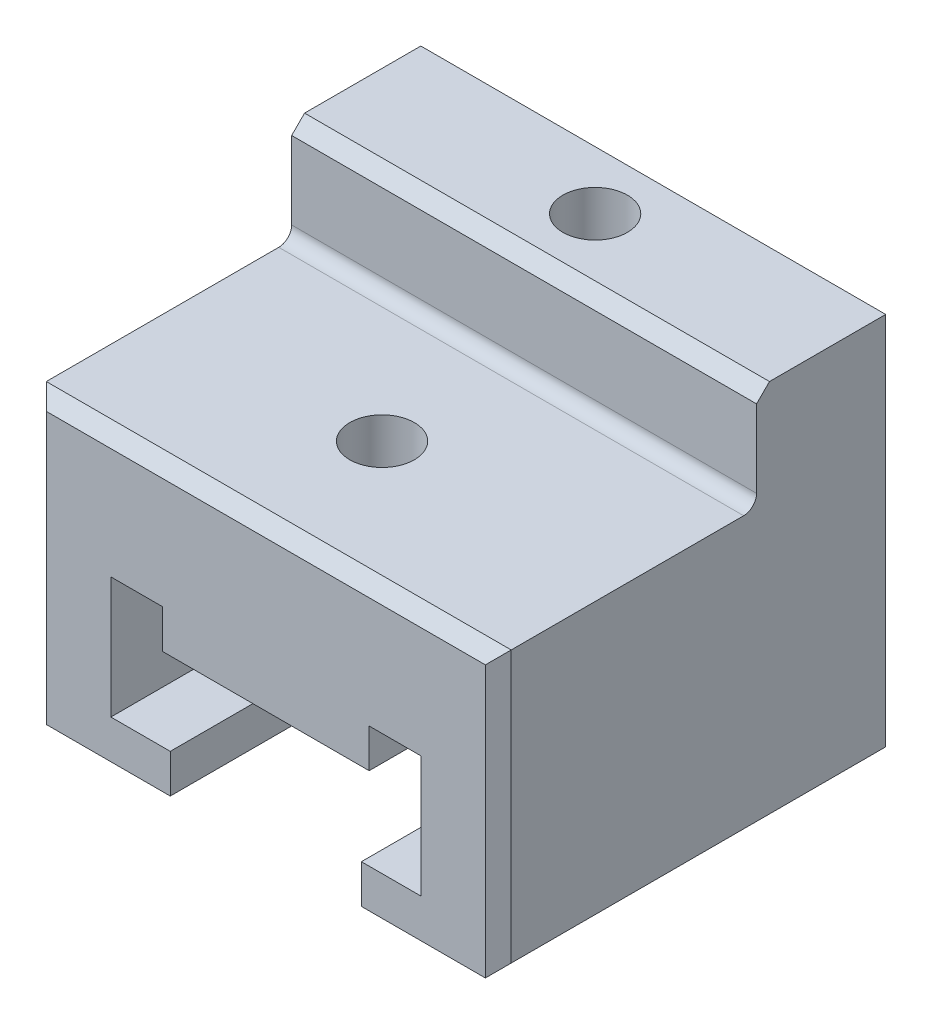
from build123d import *

# Parameters (mm, degrees)
BOSS_EXTRUDE1_START   = -14
BOSS_EXTRUDE1_DEPTH   = 15.5
SKETCH2_W             = 10
SKETCH2_H             = 4
CUT_EXTRUDE1_DEPTH    = 37.060227398
M3_TAPPED_HOLE1_D     = 2.5
M3_TAPPED_HOLE1_DEPTH = 8.5
M3_TAPPED_HOLE1_TIP   = 0.751075774
M3_TAPPED_HOLE2_D     = 2.5
CHAMFER1_SIZE         = 0.5
FILLET1_R             = 0.5


with BuildPart() as part:
    # Sketch1 → Boss-Extrude1 (new body)
    with BuildSketch(Plane.XY.offset(BOSS_EXTRUDE1_START)):
        Polygon((-3.7, -3.2), (-3.7, -4.7), (-9, -4.7), (-9, 10.3), (9, 10.3), (9, -4.7), (3.7, -4.7), (3.7, -3.2), (6, -3.2), (6, 1.5), (4, 1.5), (4, 0), (0, 0), (-4, 0), (-4, 1.5), (-6, 1.5), (-6, -3.2), align=None)
    extrude(amount=-BOSS_EXTRUDE1_DEPTH)

    # Sketch2 → Cut-Extrude1 (cut, through all)
    with BuildSketch(Plane(origin=(9, 0, 0), x_dir=(0, 0, -1), z_dir=(1, 0, 0))):
        with Locations((19, 8.3)):
            Rectangle(SKETCH2_W, SKETCH2_H)
    extrude(amount=-CUT_EXTRUDE1_DEPTH, mode=Mode.SUBTRACT)

    # M3 Tapped Hole1
    with Locations(Plane(origin=(0, 6.3, 0), x_dir=(1, 0, 0), z_dir=(0, 1, 0))):
        with Locations((-0.5, 19)):
            Hole(M3_TAPPED_HOLE1_D / 2, depth=M3_TAPPED_HOLE1_DEPTH)
            with Locations((0, 0, -(M3_TAPPED_HOLE1_DEPTH + M3_TAPPED_HOLE1_TIP / 2))):  # 118° drill point
                Cone(0, M3_TAPPED_HOLE1_D / 2, M3_TAPPED_HOLE1_TIP, mode=Mode.SUBTRACT)

    # M3 Tapped Hole2 (through all)
    with Locations(Plane(origin=(0, 10.3, 0), x_dir=(1, 0, 0), z_dir=(0, 1, 0))):
        with Locations((0, 26.75)):
            Hole(M3_TAPPED_HOLE2_D / 2)

    # Chamfer1
    chamfer1_edges = [part.edges().sort_by_distance(p)[0] for p in [
        (0, 10.3, -29.5),
        (-9, 2.8, -29.5),
        (-9, 0.8, -14),
        (9, 0.8, -14),
        (-9, -4.7, -21.75),
        (9, -4.7, -21.75),
        (0, 6.3, -14),
        (0, 10.3, -24),
        (9, 2.8, -29.5),
    ]]
    chamfer(chamfer1_edges, length=CHAMFER1_SIZE)

    # Fillet1
    fillet1_edges = [part.edges().sort_by_distance(p)[0] for p in [
        (0, 6.3, -24),
    ]]
    fillet(fillet1_edges, radius=FILLET1_R)


solid = part.part
